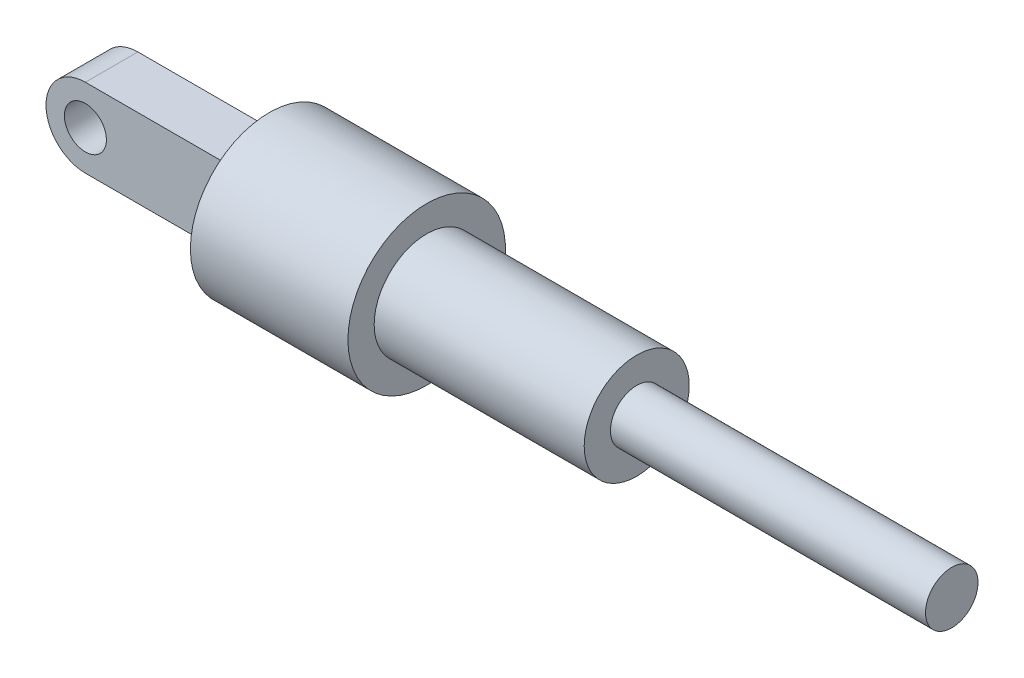
SolidWorks part; units mm, degrees
ref_plane "Front Plane" through (0, 0, 0) normal (0, 0, 1) x (1, 0, 0)
ref_plane "Top Plane" through (0, 0, 0) normal (0, 1, 0) x (1, 0, 0)
ref_plane "Right Plane" through (0, 0, 0) normal (1, 0, 0) x (0, 0, -1)
sketch "Sketch1" plane through (0, 0, 0) normal (0, 0, 1) x (1, 0, 0)
  line L0 (0, -60.0721) -> (0, 2943.5314) construction
  line L1 (0, 0) -> (0, 1.5)
  line L2 (0, 1.5) -> (3, 1.5)
  line L3 (3, 1.5) -> (3, 1)
  line L4 (3, 1) -> (13, 1)
  line L5 (13, 1) -> (13, 0)
  line L6 (0.1244, 0) -> (3003.7278, 0) construction
  line L7 (0, 0) -> (13, 0)
  point P8 (3, 1.25)
  dimension "D1" = 3
  dimension "D2" = 10
  dimension "D3" = 3
  dimension "D4" = 2
revolve "Revolve1" add sketch "Sketch1" angle 360 about L6
sketch "Sketch2" plane through (0, 0, 0) normal (0, 0, 1) x (1, 0, 0)
  line L0 (0, 0) -> (-50000, 0) construction
  line L1 (0, 0.75) -> (0, -0.75)
  line L2 (0, 1.5) -> (0, -1.5) construction
  line L3 (0, -0.75) -> (-3, -0.75)
  line L4 (0, 0) -> (0, 50000) construction
  line L5 (0, 0.75) -> (-3, 0.75)
  arc A0 (-3, -0.75) -> (-3, 0.75) centre (-3, 0) cw
  circle A1 centre (-3, 0) radius 0.4
  point P9 (0, 0)
  dimension "D1" = 0.75
  dimension "D3" = 0.8
  dimension "D2" = 3
extrude "Boss-Extrude1" add sketch "Sketch2" along normal mid plane 1
sketch "Sketch3" plane through (0, 0, 0) normal (0, 0, 1) x (1, 0, 0)
  line L0 (-1, 0.75) -> (-1, -0.75)
  line L1 (0, 0.75) -> (-3, 0.75) construction
  line L2 (-3, -0.75) -> (0, -0.75) construction
  line L3 (-1, -0.75) -> (-3, -0.75)
  line L4 (-3, 0.75) -> (-1, 0.75)
  line L5 (0, 1.5) -> (0, -1.5) construction
  arc A0 (-3, -0.75) -> (-3, 0.75) centre (-3, 0) cw
  dimension "D1" = 1
sketch "Sketch4" plane through (13, 0, 0) normal (1, 0, 0) x (0, 0, -1)
  circle A0 centre (0, 0) radius 0.5
  circle A1 centre (0, 0) radius 1
extrude "Cut-Extrude3" cut sketch "Sketch4" against normal blind 6
